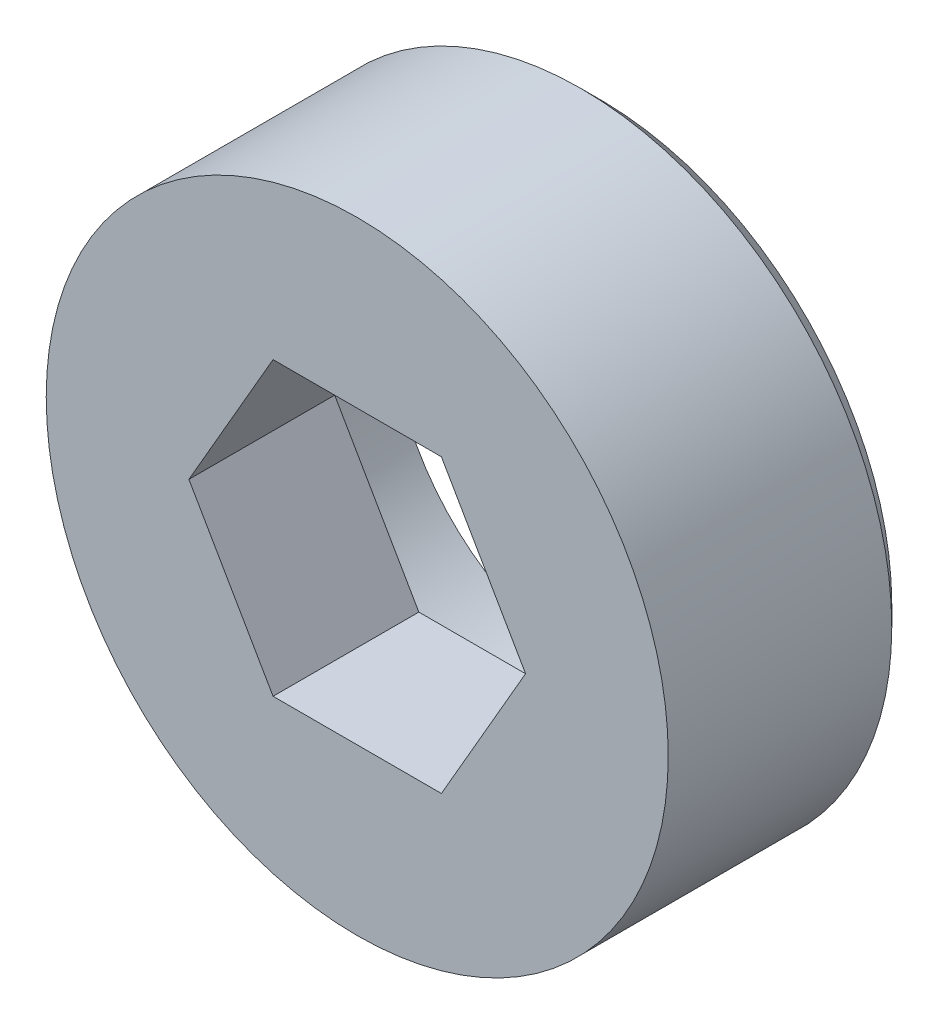
SolidWorks part; units mm, degrees
material "Q345 "
ref_plane "前视基准面" through (0, 0, 0) normal (0, 0, 1) x (1, 0, 0)
ref_plane "上视基准面" through (0, 0, 0) normal (0, 1, 0) x (1, 0, 0)
ref_plane "右视基准面" through (0, 0, 0) normal (1, 0, 0) x (0, 0, -1)
sketch "草图1" plane through (0, 0, 0) normal (0, 0, 1) x (1, 0, 0)
  circle A0 centre (0, 0) radius 32
  dimension "D1" = 64
extrude "凸台-拉伸1" add sketch "草图1" along normal blind 25
cosmetic thread "装饰螺纹线1" parameters "D2"=57.505
sketch "草图2" plane through (0, 0, 25) normal (0, 0, 1) x (1, 0, 0)
  line L0 (0, 0) -> (17.3205, 0) construction
  line L1 (17.3205, 0) -> (8.6603, 15)
  line L2 (8.6603, 15) -> (-8.6603, 15)
  line L3 (-8.6603, 15) -> (-17.3205, 0)
  line L4 (-17.3205, 0) -> (-8.6603, -15)
  line L5 (-8.6603, -15) -> (8.6603, -15)
  line L6 (8.6603, -15) -> (17.3205, 0)
  circle A0 centre (0, 0) radius 15 construction
  dimension "D1" = 30
extrude "切除-拉伸1" cut sketch "草图2" against normal through all
sketch "草图3" plane through (0, 0, 0) normal (0, 0, -1) x (-1, 0, 0)
  circle A0 centre (0, 0) radius 21.5
  dimension "D1" = 43
extrude "切除-拉伸2" cut sketch "草图3" against normal blind 10
chamfer "倒角1" distance 2 angle 45 1 edges at (32, 0, 0)
